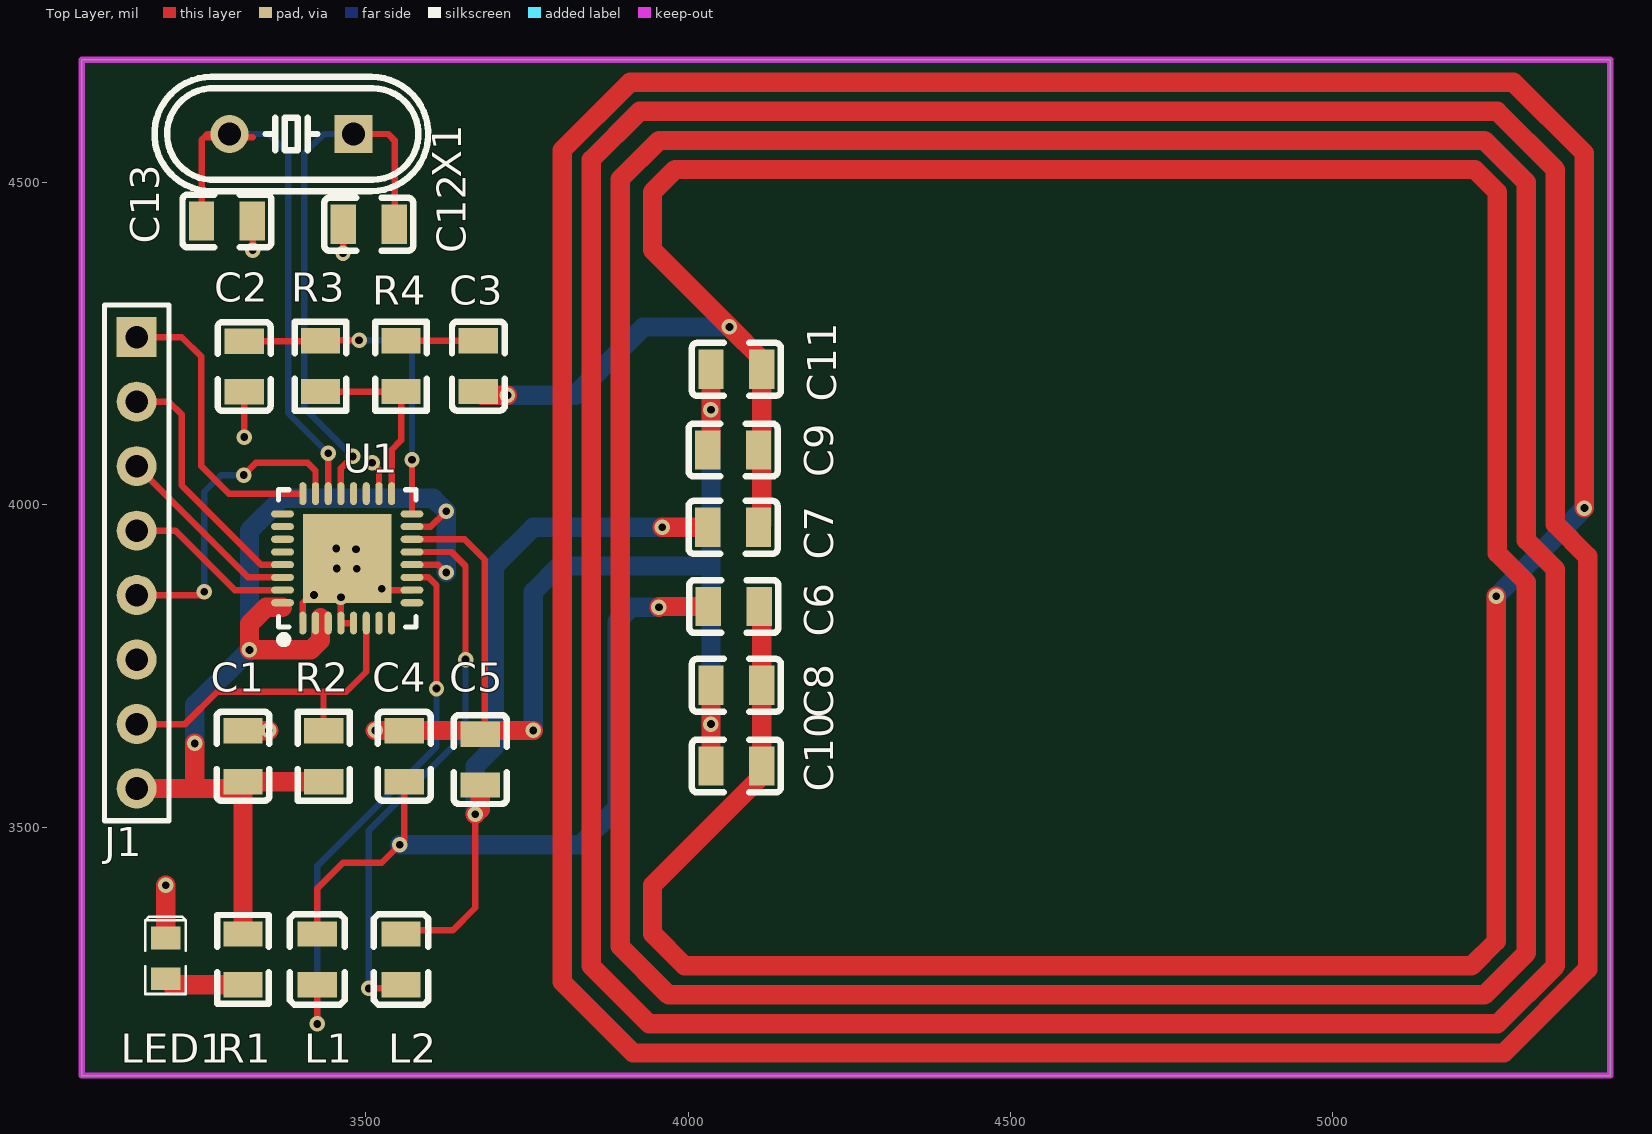
[diagram p0: Top Layer view]
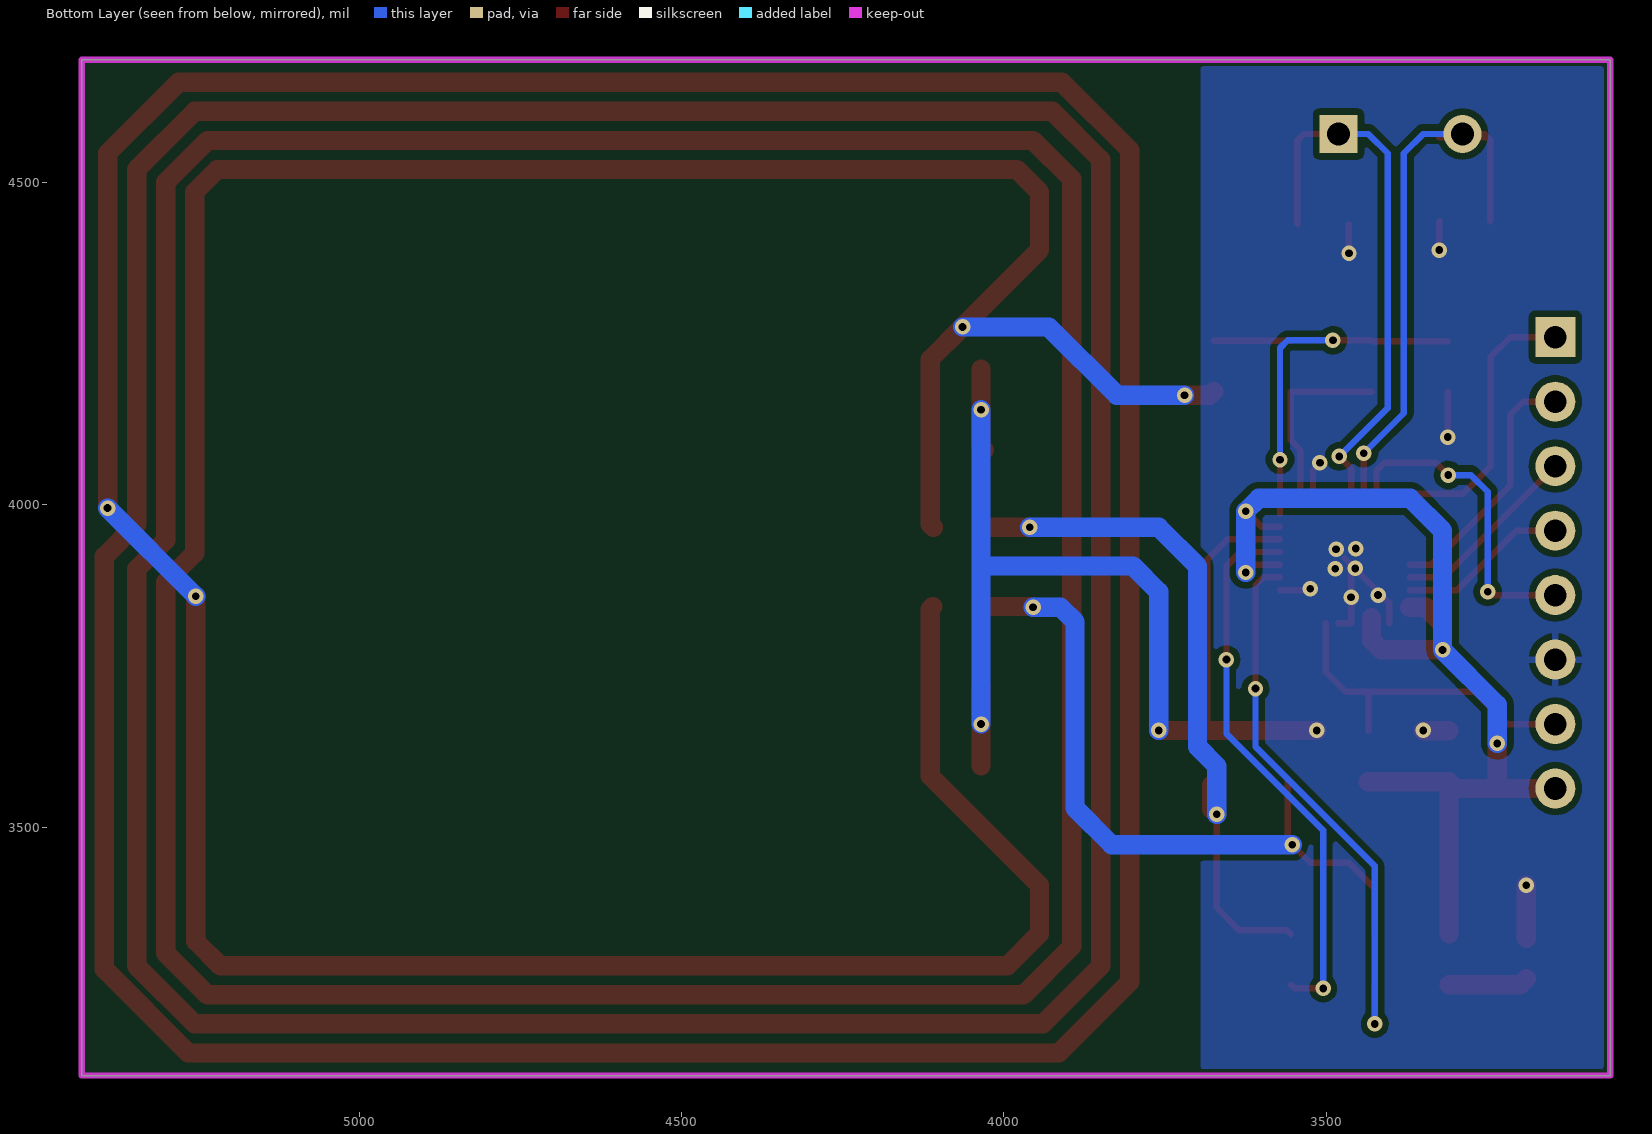
[diagram p1: Bottom Layer view, seen from below]
# Altium PCB MISC61972.pcbdoc
Units mil, origin at the board's own origin, x right, y up, seen from the top; angles counter-clockwise.
Board outline 2370 x 1575 mil, 2 copper layers (Top Layer, Bottom Layer), stack 62.206 mil thick; 23 components, 19 nets, 83 pads, 39 vias.

## Layer stack, top to bottom
Top Solder Mask Layer: solder mask 0.394, Dk 3.3
Top Layer: signal copper 1.379
Dielectric1: surface 59.449, FR4, Dk 4.5
Bottom Layer: signal copper 1.378
Bottom Solder Mask Layer: solder mask 0.394, Dk 3.3

## Board outline
3060,4690 3060,3115 5430,3115 5430,4690

## Design rules (kind name [scope] priority, off if disabled: settings)
BoardOutlineClearance copperThickness2oz_1 [All] p2 off: genericclearance=7.99 ignorepadtopadclearanceinfootprint=FALSE except(0: Arc-SplitContinuation Track-SplitContinuation SMDPad-SplitContinuation THPad-SplitContinuation Via-SplitContinuation Fill-SplitContinuation Region-SplitContinuation Poly-SplitContinuation Text-SplitContinuation Hole-SplitContinuation; 5.98: Arc-CutoutEdge SMDPad-CutoutEdge THPad-CutoutEdge Via-CutoutEdge Fill-CutoutEdge Region-CutoutEdge Text-CutoutEdge; 6.93: Hole-OutlineEdge Hole-CutoutEdge; 10: Poly-OutlineEdge Poly-CutoutEdge; 11.81: Arc-OutlineEdge Track-OutlineEdge SMDPad-OutlineEdge THPad-OutlineEdge Via-OutlineEdge Fill-OutlineEdge Region-OutlineEdge Text-OutlineEdge Track-CutoutEdge)
BoardOutlineClearance copperThickness1oz_1 [All] p4: genericclearance=4.02 ignorepadtopadclearanceinfootprint=FALSE except(0: Arc-SplitContinuation Track-SplitContinuation SMDPad-SplitContinuation THPad-SplitContinuation Via-SplitContinuation Fill-SplitContinuation Region-SplitContinuation Poly-SplitContinuation Text-SplitContinuation Hole-SplitContinuation; 6: SMDPad-CutoutEdge THPad-CutoutEdge Via-CutoutEdge Fill-CutoutEdge Region-CutoutEdge Text-CutoutEdge; 6.93: Hole-OutlineEdge Hole-CutoutEdge; 10: Poly-OutlineEdge Poly-CutoutEdge; 11.8: Arc-OutlineEdge Track-OutlineEdge SMDPad-OutlineEdge THPad-OutlineEdge Via-OutlineEdge Fill-OutlineEdge Region-OutlineEdge Text-OutlineEdge; 11.81: Arc-CutoutEdge Track-CutoutEdge)
Clearance copperThickness2oz [All] p1 off: gap=7.99 ignorepadtopadclearanceinfootprint=FALSE except(5.98: SMDPad-Track SMDPad-SMDPad THPad-Track SMDPad-THPad THPad-THPad Track-Via SMDPad-Via THPad-Via Via-Via Fill-Track Region-Track Fill-SMDPad Region-SMDPad Fill-THPad Region-THPad Fill-Via Region-Via Fill-Fill Fill-Region Region-Region Arc-Track Arc-SMDPad Arc-THPad Arc-Via Fill-Arc Region-Arc Arc-Arc Text-Track SMDPad-Text Text-THPad Text-Via Fill-Text Region-Text Arc-Text Text-Text; 6.93: Hole-Track Hole-SMDPad Hole-THPad Hole-Via Fill-Hole Region-Hole Hole-Arc Hole-Text; 10: Poly-Track Poly-SMDPad Poly-THPad Poly-Via Poly-Fill Poly-Region Poly-Poly Poly-Arc Poly-Text Poly-Hole)
Clearance copperThickness1oz [All] p3: gap=4.02 ignorepadtopadclearanceinfootprint=FALSE except(5.98: SMDPad-Track SMDPad-SMDPad THPad-Track SMDPad-THPad THPad-THPad Track-Via SMDPad-Via THPad-Via Via-Via Fill-Track Region-Track Fill-SMDPad Region-SMDPad Fill-THPad Region-THPad Fill-Via Region-Via Fill-Fill Fill-Region Region-Region; 6: Arc-Track Arc-SMDPad Arc-THPad Arc-Via Fill-Arc Region-Arc Arc-Arc Text-Track SMDPad-Text Text-THPad Text-Via Fill-Text Region-Text Arc-Text Text-Text; 6.93: Hole-Track Hole-SMDPad Hole-THPad Hole-Via Fill-Hole Region-Hole Hole-Arc Hole-Text; 10: Poly-Track Poly-SMDPad Poly-THPad Poly-Via Poly-Fill Poly-Region Poly-Poly Poly-Arc Poly-Text Poly-Hole)
Creepage creepage [All] p1: checkdistance=0 ignoreinternallayers=TRUE applytopolygonpour=TRUE
DiffPairsRouting differentialPair [All] p1: maxlimit=6 minlimit=6 mostfreqgap=6 toplayer_minwidth=5 toplayer_prefwidth=10 toplayer_maxwidth=100 toplayer_mingap=6 toplayer_prefgap=6 toplayer_maxgap=6 bottomlayer_minwidth=5 bottomlayer_prefwidth=10 bottomlayer_maxwidth=100 bottomlayer_mingap=6 bottomlayer_prefgap=6 bottomlayer_maxgap=6 maxuncoupledlength=10
HoleToHoleClearance otherClearance [All] p1: gap=11.81 allowstackedmicrovias=TRUE
Length netLength [All] p1: minlimit=0 maxlimit=0
MatchedLengths netLengthTolerance [All] p1: tolerance=1000
PasteMaskExpansion pasteMaskExpansion [All] p1: expansion=0
PlaneConnect innerPlane [All] p1: planeconnectstyle=Relief reliefexpansion=20 reliefentries=4 reliefconductorwidth=10 reliefairgap=10
PolygonConnect copperRegion [All] p1: connectstyle=Relief reliefconductorwidth=10 reliefentries=4 polygonreliefangle="90 Angle" airgapwidth=10 via.connectstyle=Relief via.reliefconductorwidth=10 via.reliefentries=4 via.polygonreliefangle="90 Angle" via.airgapwidth=10
RoutingVias viaSize [All] p1: holewidth=12.01 width=24.02 viastyle="Through Hole" minholewidth=11.81 minwidth=19.68 maxholewidth=248.03 maxwidth=393.7
SolderMaskExpansion solderMaskExpansion [IsVia] p1: expansion=-1000 istentingtop=TRUE
SolderMaskExpansion solderMaskExpansion [All] p2: expansion=2 istentingtop=FALSE
Width copperThickness2oz_2 [All] p1 off: maxlimit=100 minlimit=8 preferedwidth=10
Width copperThickness1oz_2 [All] p2: maxlimit=100 minlimit=5 preferedwidth=10

## Components (designator, comment, footprint, x,y, rotation, side; value= is the part's Value field where it differs from the comment)
C1 "0.1u" C0805 3310,3610 r270 top
C2 "0.1u" C0805 3311.7,4214.41 r90 top
C3 "0.1u" C0805 3675,4215 r270 top
C4 "47P" C0805 3560,3610 r270 top
C5 "47P" C0805 3677.88,3604.93 r90 top
C6 "15P" C0805 4071,3842.2 r0 top
C7 "15P" C0805 4070,3965 r0 top
C8 "10pf" C0805 4075,3720 r0 top
C9 "10pf" C0805 4070,4085 r180 top
C10 "180P" C0805 4075,3595 r0 top
C11 "180P" C0805 4075,4210 r180 top
C12 "15P" C0805 3505,4435 r180 top
C13 "15P" C0805 3285,4440 r0 top
J1 "HDR-M-2.54_1x8" HDR-M-2.54_1X8 3145,3860 r270 top
L1 "2.2uH" L0805 3425,3295 r90 top
L2 "2.2uH" L0805 3555,3295 r90 top
LED1 "LED-0805_G" LED-0805_G 3190,3265 r270 top
R1 "1k" R0805 3310,3295 r270 top
R2 "10K" R0805 3435,3610 r90 top
R3 "820" R0805 3430,4215 r270 top
R4 "5.1k" R0805 3555,4215 r90 top
U1 "MF522 COPY" LC-QFN-32_5X5X05P 3465,3910 r0 top
X1 "27.12MHz" HC-49US_L11.5-W4.5-P4.88 3385,4575 r180 top

## Footprints (in the part's own frame and the unit in brackets; to place one, negate y for a bottom-side part, rotate by r counter-clockwise, add the part's x,y. Pads: shape width x height; smd on the part's side, far side on the other; paste and mask are expansions set on the pad)
C0805 [mm]
  rect 1x1.55 smd paste+0 mask+0.102: 1(-1,0) 2(1,0)
  silkscreen extent -1.75,-1.04 1.75,1.04
HC-49US_L11.5-W4.5-P4.88 [mm]
  rect 1.5x1.5 hole 0.9 paste+0 mask+0.051: 1(-2.44,0)
  round 1.5 hole 0.9 paste+0 mask+0.051: 2(2.44,0)
  silkscreen extent -5.39,-2.25 5.39,2.25
HDR-M-2.54_1X8 [mil]
  rect 62x62 hole 35 paste+0 mask+2: 1(-400,0)
  round 62 hole 35 paste+0 mask+2: 2(-300,0) 3(-200,0) 4(-100,0) 5(0,0) 6(100,0) 7(200,0) 8(300,0)
  silkscreen extent -450,-50 350,50
L0805 [mm]
  rect 1x1.55 smd paste+0 mask+0.102: 1(-1,0) 2(1,0)
  silkscreen extent -1.78,-1.08 1.78,1.08
LC-QFN-32_5X5X05P [mil]
  rect 137.8x137.8 smd paste+0 mask+2: 0(6.6,6.96)
  oval 11.02x35.43 smd paste+0 mask+2: 1(-62.3,-93.43) 2(-42.61,-93.43) 3(-22.93,-93.43) 4(-3.24,-93.43) 5(16.44,-93.43) 6(36.13,-93.43) 7(55.81,-93.43) 8(75.5,-93.43) 17(75.5,107.35) 18(55.81,107.35) 19(36.13,107.35) 20(16.44,107.35) 21(-3.24,107.35) 22(-22.93,107.35) 23(-42.61,107.35) 24(-62.3,107.35)
  oval 35.43x11.02 smd paste+0 mask+2: 9(107,-61.94) 10(107,-42.25) 11(107,-22.57) 12(107,-2.88) 13(107,16.8) 14(107,36.49) 15(107,56.17) 16(107,75.86) 25(-93.79,75.86) 26(-93.79,56.17) 27(-93.79,36.49) 28(-93.79,16.8) 29(-93.79,-2.88) 30(-93.79,-22.57) 31(-93.79,-42.25) 32(-93.79,-61.94)
  silkscreen extent -100,-125 113,113
LED-0805_G [mm]
  rect 0.9x1.15 smd: 1(0,0) 2(-1.6,0)
  silkscreen extent -2.45,-0.8 0.6,0.8
R0805 [mm]
  rect 1x1.55 smd paste+0 mask+0.102: 1(-1,0) 2(1,0)
  silkscreen extent -1.75,-1.02 1.75,1.02

## Via types
v1: diameter 24.02, hole 12, Top Layer to Bottom Layer, 39 vias

## Nets (pads, with @x,y where several pads share a name; then routed paths per layer and width w, separated by ;. In a path a pad name is that pad's centre, name@x,y a point inside that pad or via, vN(x,y) a via of type N, cw(c..) or ccw(c..) an arc to the next point about the centre after c; other vN are vias at no path point)
3.3V: C1.2 J1.8 R1.1 R2.1 U1.2 U1.3 U1.12 U1.15 U1.32 | length 1769.3
  Top Layer w10: U1.12 3612.88,3907.12 v1(3625,3895) ; U1.15 3601.17,3966.17 v1(3625,3990)
  Top Layer w30: J1.8 3234.43,3560 ; v1(3235,3630) 3235,3560.57 3234.43,3560 ; R1.1 C1.2 ; 3371.21,3841.26 3346.26,3841.26 3320,3815 v1(3320,3775) 3415,3775 3430,3790 3430,3825 ; R2.1 C1.2 ; 3234.43,3560 3299.37,3560 C1.2
  Bottom Layer w30: v1(3235,3630) 3235,3690 v1(3320,3775) 3320,3960 3370,4010 3605,4010 v1(3625,3990) v1(3625,3895)
$1N2: LED1.1 R1.2 | length 123.9
  Top Layer w30: LED1.1 3199.37,3255.63 R1.2
$1N23: L1.1 U1.11 | length 860.4
  Top Layer w10: v1(3425,3195) L1.1 ; U1.11 3597.57,3887.43 3610,3875 v1(3610,3715)
  Bottom Layer w10: v1(3425,3195) 3425,3440 3610,3625 v1(3610,3715)
$1N24: L2.1 U1.13 | length 861.5
  Top Layer w10: v1(3505,3250) 3549.37,3250 L2.1 ; U1.13 3633.2,3926.8 3655,3905 v1(3655,3760)
  Bottom Layer w10: v1(3505,3250) 3505,3495 3655,3645 v1(3655,3760)
$1N25: R3.2 R4.1 U1.17 | length 289.3
  Top Layer w10: R3.2 R4.1 3555,4100 3540.5,4085.5 U1.17
$1N26: C2.2 R3.1 U1.16 | length 522.9
  Top Layer w10: C2.2 3429.41,4253.78 R3.1 3430.63,4255 v1(3490,4255) ; U1.16 v1(3572,4070)
  Bottom Layer w10: v1(3490,4255) 3560,4255 3572,4243 v1(3572,4070)
$1N27: C12.1 U1.21 X1.1 | length 853.1
  Top Layer w10: U1.21 3461.76,4056.76 v1(3480,4075) ; X1.1 3535,4575 3545,4565 3545,4435.63 C12.1
  Bottom Layer w10: v1(3480,4075) 3405,4150 3405,4545 3435,4575 X1.1
$1N28: C13.1 U1.22 X1.2 | length 904.7
  Top Layer w10: C13.1 3245.63,4565.63 3250,4570 ; X1.2 3255,4575 3250,4570 ; 3325,4570 3250,4570 ; U1.22 v1(3442.07,4080)
  Bottom Layer w10: X1.2 3350,4575 3380,4545 3380,4142.07 v1(3442.07,4080)
$1N29: C3.1 R4.2 | length 120
  Top Layer w10: R4.2 C3.1
$1N30: C4.2 C6.1 L1.2 | length 1128.1
  Top Layer w10: L1.2 3425,3405 3465,3445 3525,3445 3560,3480 C4.2
  Top Layer w30: v1(3955,3841.21) 3955.99,3842.2 C6.1
  Bottom Layer w30: v1(3552.93,3472.93) 3832.93,3472.93 3890,3530 3890,3818.79 3912.43,3841.21 v1(3955,3841.21)
$1N31: C5.1 C7.1 L2.2 | length 1078.6
  Top Layer w10: L2.2 3560.63,3340 3635,3340 3670,3375 v1(3670,3520)
  Top Layer w30: v1(3670,3520) 3677.88,3527.88 C5.1 ; v1(3960,3965) C7.1
  Bottom Layer w30: v1(3670,3520) 3670,3595 3700,3625 3700,3905 3760,3965 v1(3960,3965)
$1N35: C3.2 C6.2 C7.2 C8.2 C9.1 C10.2 C11.1 | length 22407.9
  Top Layer w30: C3.2 3680.63,4170 v1(3720,4170) ; C7.2 4114.37,3970.01 C11.1 4114.37,4225.63 v1(4064.21,4275.79) 3945,4395 3945,4485 3980,4520 5220,4520 5255,4485 5255,3925 5300,3880 5300,3305 5235,3240 3970,3240 3895,3315 3895,4505 3955,4565 5235,4565 5300,4500 5300,3945 5345,3900 5345,3285 5255,3195 3940,3195 3850,3285 3850,4535 3925,4610 5255,4610 5345,4520 5345,3970 5395,3920 5395,3280 5265,3150 3915,3150 3805,3260 3805,4550 3910,4655 5280,4655 5390,4545 v1(5390,3995) ; C6.2 4114.37,3838.21 C8.2 C10.2 4114.37,3579.37 3945,3410 3945,3335 3995,3285 5215,3285 5253.21,3323.21 v1(5253.21,3858.21)
  Bottom Layer w30: v1(3720,4170) 3825,4170 3930.79,4275.79 v1(4064.21,4275.79) ; v1(5253.21,3858.21) v1(5390,3995)
GND: C1.1 C2.1 C4.1 C5.2 C8.1 C9.2 C10.1 C11.2 C12.2 C13.2 J1.6 LED1.2 U1.0 U1.1 U1.4 U1.5 U1.10 U1.14 U1.18 | length 2514.4
  Top Layer w10: v1(3311.7,4105) C2.1 ; C13.2 3325,4439.37 v1(3325,4395) ; U1.1 3402.7,3848.06 U1.0@3461.76,3907.12 ; v1(3465,4390) 3465.63,4390.63 C12.2 ; U1.0 U1.0@3461.76,3907.12 ; U1.5 U1.4 v1(3461.76,3856.48) U1.0@3461.76,3907.12 ; v1(3510,4065) 3520.81,4054.19 U1.18 ; v1(3525,3870) 3527.25,3867.75 U1.10 ; U1.14 3653.51,3946.49 3685,3915 3685,3651.41 3683.59,3650 C5.2
  Top Layer w30: LED1.2 v1(3190,3410) ; C1.1 3349.37,3649.37 v1(3350,3650) ; v1(3515,3650) C4.1@3560.63,3650 ; C4.1 C4.1@3560.63,3650 ; v1(3760,3650) 3683.59,3650 C4.1@3560.63,3650 ; C9.2 4035.63,4090 v1(4035.63,4147.51) C11.2 ; C10.1 v1(4035.63,3660) C8.1
  Bottom Layer w30: v1(3760,3650) 3760,3865 3800,3905 4035.63,3905 ; v1(4035.63,3660) 4035.63,3905 ; v1(4035.63,4147.51) 4035.63,3905
  other v1: 3420,3860 3455.39,3901.22 3486.34,3900.7 3485.04,3931.14 3454.35,3932.18
IRQ: J1.5 U1.23 | length 493.5
  Top Layer w10: J1.5 3245,3860 v1(3250,3865) ; v1(3311.14,4046.14) 3330,4065 3410,4065 3422.39,4052.61 U1.23
  Bottom Layer w10: v1(3250,3865) 3250,4020 3276.14,4046.14 v1(3311.14,4046.14)
MISO: J1.4 U1.31 | length 264.4
  Top Layer w10: J1.4 3205,3960 3297.25,3867.75 U1.31
MOSI: J1.3 U1.30 | length 297.7
  Top Layer w10: J1.3 3317.57,3887.43 U1.30
RST: J1.7 R2.2 U1.6 | length 525.9
  Top Layer w10: J1.7 3220,3660 3270,3710 3434.74,3710 ; R2.2 3434.74,3649.62 3434.74,3710 ; U1.6 3501.13,3741.13 3470,3710 3434.74,3710
SCK: J1.2 U1.29 | length 395.4
  Top Layer w10: J1.2 3195,4160 3215,4140 3215,4030 3337.88,3907.12 U1.29
SDA: J1.1 U1.24 | length 457.8
  Top Layer w10: J1.1 3215,4260 3245,4230 3245,4060 3287.65,4017.35 U1.24
pads on no net: U1.7 U1.8 U1.9 U1.19 U1.20 U1.25 U1.26 U1.27 U1.28

## Polygon pours and split planes (outlines as drawn)
GND on Bottom Layer (solid, remove dead copper, pour order 2): 3000,4715 3000,3000 3695,3000 3695,4715

## Keep-outs
Board Outline Layer:
  the board outline again, w10